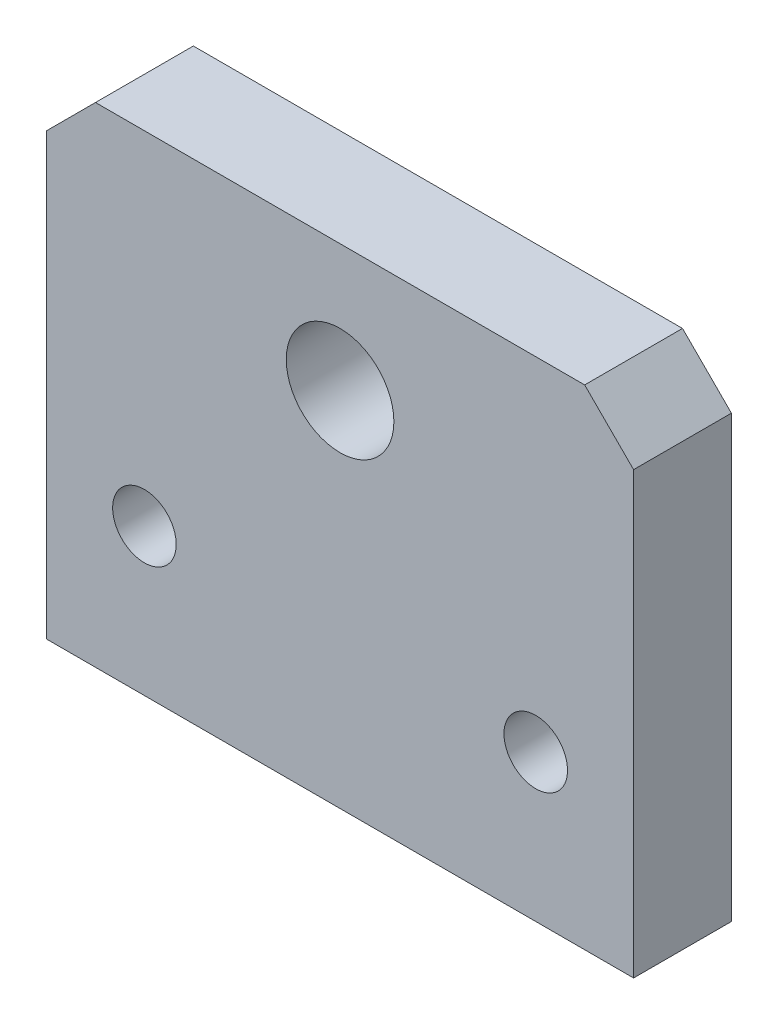
from build123d import *

# Parameters (mm, degrees)
SKETCH1_W           = 60
SKETCH1_H           = 50
BOSS_EXTRUDE1_DEPTH = 10
SKETCH2_R           = 5.5
CUT_EXTRUDE1_DEPTH  = 18
CHAMFER1_SIZE       = 5
SKETCH3_R           = 3.25
CUT_EXTRUDE2_DEPTH  = 46.967787324


with BuildPart() as part:
    # Sketch1 → Boss-Extrude1 (new body)
    with BuildSketch(Plane.XY):
        with Locations((-5.243851729, -2.76523702)):
            Rectangle(SKETCH1_W, SKETCH1_H)
    extrude(amount=BOSS_EXTRUDE1_DEPTH)

    # Sketch2 → Cut-Extrude1 (cut)
    with BuildSketch(Plane(origin=(0, 0, 0), x_dir=(-1, 0, 0), z_dir=(0, 0, -1))):
        with Locations((5.243851729, 9.23476298)):
            Circle(SKETCH2_R)
    extrude(amount=-CUT_EXTRUDE1_DEPTH, mode=Mode.SUBTRACT)

    # Chamfer1
    chamfer1_edges = [part.edges().sort_by_distance(p)[0] for p in [
        (-35.243851729, 22.23476298, 5),
        (24.756148271, 22.23476298, 5),
    ]]
    chamfer(chamfer1_edges, length=CHAMFER1_SIZE)

    # Sketch3 → Cut-Extrude2 (cut, through all)
    with BuildSketch(Plane(origin=(0, 0, 0), x_dir=(-1, 0, 0), z_dir=(0, 0, -1))):
        with Locations((-14.756148271, -12.76523702)):
            Circle(SKETCH3_R)
        with Locations((25.243851729, -12.76523702)):
            Circle(SKETCH3_R)
    extrude(amount=-CUT_EXTRUDE2_DEPTH, mode=Mode.SUBTRACT)


solid = part.part
